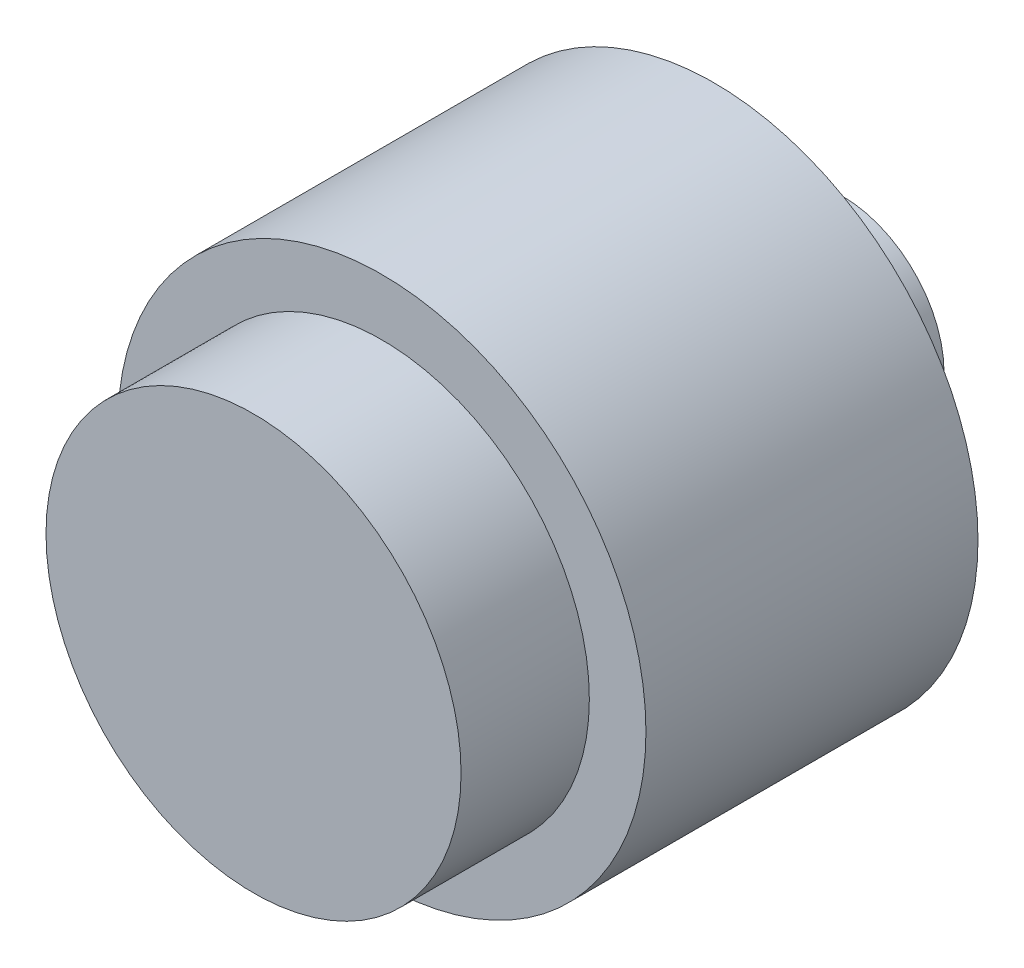
from build123d import *

# Parameters (mm, degrees)
SKETCH1_R           = 27
BOSS_EXTRUDE1_DEPTH = 34
SKETCH2_R           = 70
BOSS_EXTRUDE2_DEPTH = 88
SKETCH3_R           = 55
BOSS_EXTRUDE3_DEPTH = 34


with BuildPart() as part:
    # Sketch1 → Boss-Extrude1 (new body)
    with BuildSketch(Plane.XY):
        Circle(SKETCH1_R)
    extrude(amount=BOSS_EXTRUDE1_DEPTH)

    # Sketch2 → Boss-Extrude2 (add)
    with BuildSketch(Plane.XY.offset(34)):
        Circle(SKETCH2_R)
    extrude(amount=BOSS_EXTRUDE2_DEPTH)

    # Sketch3 → Boss-Extrude3 (add)
    with BuildSketch(Plane.XY.offset(122)):
        Circle(SKETCH3_R)
    extrude(amount=BOSS_EXTRUDE3_DEPTH)


solid = part.part
